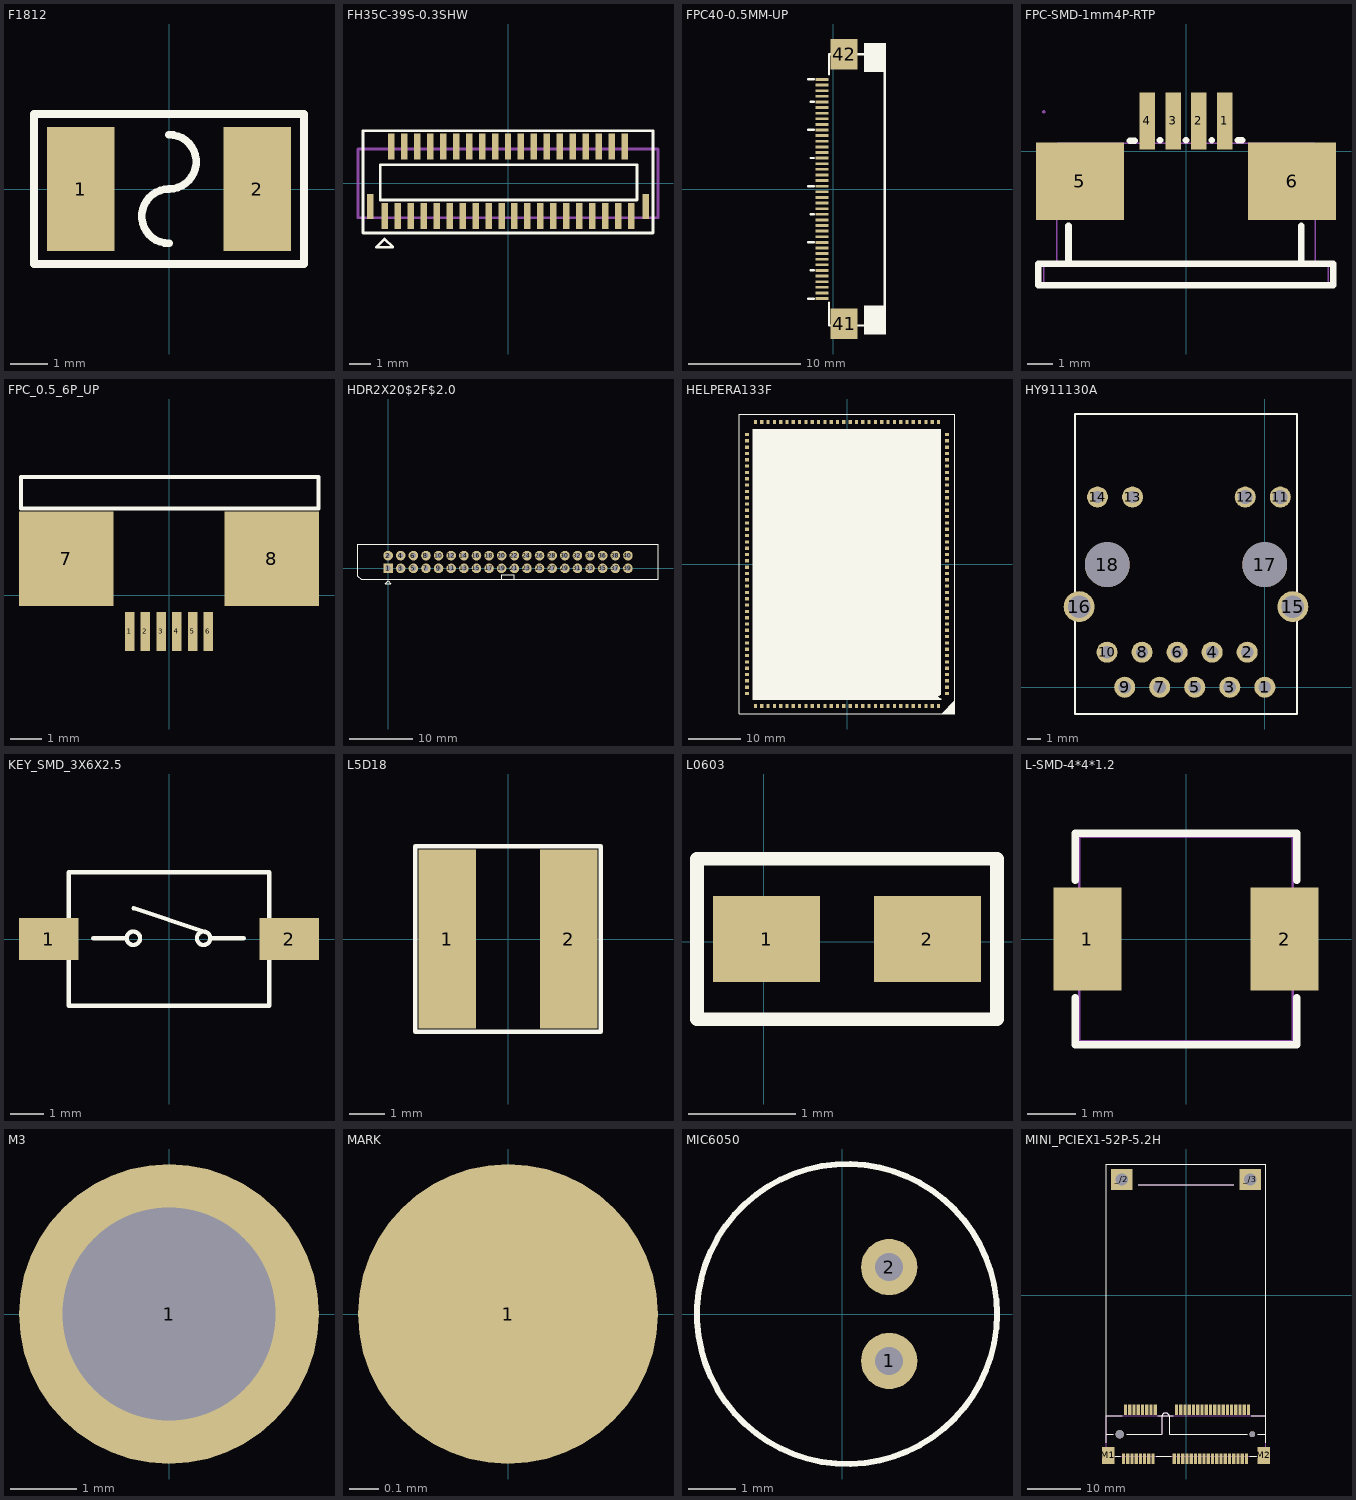
[diagram p0: the footprints below, top view; thin cyan lines are the x and y axes]
# Altium footprint library MISC82162-2.PcbLib: 66 footprints (part 2 of 5)
Each footprint in its own frame and in the unit in brackets; x right, y up, seen from the top. Pads: shape width x height; smd on the part's side, far side on the other; paste and mask are expansions set on the pad; w line width, h text height; cw(c..) or ccw(c..) is an arc to the next point about the centre after c.

## F1812 [mm]
pads (2):
  rect 1.8x3.3 smd: 1(-2.349,0) 2(2.349,0)
Top Overlay:
  lines w0.203: 0,-1.45 cw(c0,-0.725) 0,0 ccw(c0,0.725) 0,1.45 ; -3.6,-2 -3.6,2 3.6,2 3.6,-2 -3.6,-2

## FH35C-39S-0.3SHW [mm]
pads (41):
  rect 0.3x1.2 smd: 1(-5.7,-1.5) 2(-5.4,1.7) 3(-5.1,-1.5) 4(-4.8,1.7) 5(-4.5,-1.5) 6(-4.2,1.7) 7(-3.9,-1.5) 8(-3.6,1.7) 9(-3.3,-1.5) 10(-3,1.7) 11(-2.7,-1.5) 12(-2.4,1.7) 13(-2.1,-1.5) 14(-1.8,1.7) 15(-1.5,-1.5) 16(-1.2,1.7) 17(-0.9,-1.5) 18(-0.6,1.7) 19(-0.3,-1.5) 20(0,1.7) 21(0.3,-1.5) 22(0.6,1.7) 23(0.9,-1.5) 24(1.2,1.7) 25(1.5,-1.5) 26(1.8,1.7) 27(2.1,-1.5) 28(2.4,1.7) 29(2.7,-1.5) 30(3,1.7) 31(3.3,-1.5) 32(3.6,1.7) 33(3.9,-1.5) 34(4.2,1.7) 35(4.5,-1.5) 36(4.8,1.7) 37(5.1,-1.5) 38(5.4,1.7) 39(5.7,-1.5)
  rect 0.3x1.15 smd: 40(6.35,-1.062) 41(-6.35,-1.062)
Top Overlay:
  lines w0.127: -6.7,-2.29 -6.7,2.427 6.7,2.427 6.7,-2.29 -6.7,-2.29 ; -6.08,-2.942 -5.699,-2.561 -5.318,-2.943 -6.068,-2.943 -6.08,-2.942 ; -5.9,-0.768 5.96,-0.768 5.96,0.863 -5.9,0.863 -5.9,-0.768
Mechanical 18:
  lines w0.127: -6.925,-1.587 6.925,-1.587 6.925,1.587 -6.925,1.587 -6.925,-1.587

## FPC40-0.5MM-UP [mm]
pads (42):
  rect 1.15x0.25 smd: 1(-0.984,9.75) 2(-0.984,9.25) 3(-0.984,8.75) 4(-0.984,8.25) 5(-0.984,7.75) 6(-0.984,7.25) 7(-0.984,6.75) 8(-0.984,6.25) 9(-0.984,5.75) 10(-0.984,5.25) 11(-0.984,4.75) 12(-0.984,4.25) 13(-0.984,3.75) 14(-0.984,3.25) 15(-0.984,2.75) 16(-0.984,2.25) 17(-0.984,1.75) 18(-0.984,1.25) 19(-0.984,0.75) 20(-0.984,0.25) 21(-0.984,-0.25) 22(-0.984,-0.75) 23(-0.984,-1.25) 24(-0.984,-1.75) 25(-0.984,-2.25) 26(-0.984,-2.75) 27(-0.984,-3.25) 28(-0.984,-3.75) 29(-0.984,-4.25) 30(-0.984,-4.75) 31(-0.984,-5.25) 32(-0.984,-5.75) 33(-0.984,-6.25) 34(-0.984,-6.75) 35(-0.984,-7.25) 36(-0.984,-7.75) 37(-0.984,-8.25) 38(-0.984,-8.75) 39(-0.984,-9.25) 40(-0.984,-9.75)
  rect 2.4x2.7 smd: 41(0.984,-12) 42(0.984,12)
Top Overlay:
  region: 2.801,-12.924 4.706,-12.924 4.706,-10.384 2.801,-10.384
  region: 2.801,10.444 4.706,10.444 4.706,12.984 2.801,12.984
  lines w0.203: -2.218,-9.761 -1.713,-9.761 ; -2.218,-4.746 -1.713,-4.746 ; -2.218,0.253 -1.713,0.253 ; -2.218,5.262 -1.713,5.262 ; -2.218,9.756 -1.713,9.756 ; -2,-7.241 -1.713,-7.241 ; -2,-2.242 -1.713,-2.242 ; -2,2.767 -1.713,2.767 ; -2,7.769 -1.713,7.769 ; -0.367,-10.106 -0.367,-12.153 4.604,-12.153 4.604,11.992 -0.367,11.992 -0.367,10.189
Top Paste:
  lines w0.152: -0.349,-10.65 -0.349,-12.153 1.316,-12.153

## FPC-SMD-1mm4P-RTP [mm]
pads (6):
  rect 0.6x2.2 smd: 1(1.499,1.163) 2(0.499,1.163) 3(-0.5,1.163) 4(-1.5,1.163)
  rect 3.4x3 smd: 5(-4.1,-1.162) 6(4.1,-1.163)
Top Overlay:
  lines w0.254: -5.718,-5.192 4.48,-5.192 ; -5.718,-5.19 -5.718,-4.36 ; -5.718,-4.352 5.69,-4.352 ; -4.543,-4.352 -4.543,-2.893 ; -2.175,0.4 -1.988,0.4 ; -1.004,0.415 -0.995,0.415 ; -0.004,0.415 0.004,0.415 ; 0.995,0.415 1.004,0.415 ; 1.995,0.415 2.182,0.415 ; 4.456,-4.352 4.456,-2.894 ; 4.49,-5.192 5.69,-5.192 5.69,-4.362
Mechanical 6:
  circle w0.2: c1.525,1.975 r0.1
Mechanical 15:
  region: 5,-2.413 3.2,-2.413 3.2,0.087 5,0.087
  region: -3.2,-2.412 -5,-2.412 -5,0.088 -3.2,0.088
  region: -1.625,1.512 -1.375,1.512 -1.375,0.112 -1.625,0.112
  region: -0.625,1.512 -0.375,1.512 -0.375,0.112 -0.625,0.112
  region: 1.374,1.512 1.624,1.512 1.624,0.112 1.374,0.112
  region: 0.374,1.512 0.625,1.512 0.625,0.112 0.374,0.112
  region: -5.44,1.512 -5.44,1.537 -5.475,1.572 -5.525,1.572 -5.56,1.537 -5.56,1.512 -5.56,1.488 -5.525,1.452 -5.475,1.452 -5.44,1.488
  lines w0.051: -5.5,-5.2 5.5,-5.2 5.5,-4.35 5,-4.35 5,0.3 -5,0.3 -5,-4.325 -5.5,-4.325 -5.5,-5.2

## FPC_0.5_6P_UP [mm]
pads (8):
  rect 0.3x1.25 smd: 1(-1.25,-1.15) 2(-0.75,-1.15) 3(-0.25,-1.15) 4(0.25,-1.15) 5(0.75,-1.15) 6(1.25,-1.15)
  rrect0% 3x3 smd: 7(-3.25,1.15) 8(3.25,1.15)
Top Overlay:
  lines w0.127: -4.691,2.75 4.737,2.75 4.737,3.75 -4.691,3.75 -4.691,2.75

## HDR2X20$2F$2.0 [mil]
pads (40):
  rect 60x60 hole 32: 1(0,0)
  round 60 hole 32: 2(0,78.74) 3(78.74,0) 4(78.74,78.74) 5(157.48,0) 6(157.48,78.74) 7(236.22,0) 8(236.22,78.74) 9(314.96,0) 10(314.96,78.74) 11(393.7,0) 12(393.7,78.74) 13(472.44,0) 14(472.44,78.74) 15(551.18,0) 16(551.18,78.74) 17(629.92,0) 18(629.92,78.74) 19(708.66,0) 20(708.66,78.74) 21(787.4,0) 22(787.4,78.74) 23(866.14,0) 24(866.14,78.74) 25(944.88,0) 26(944.88,78.74) 27(1023.62,0) 28(1023.62,78.74) 29(1102.36,0) 30(1102.36,78.74) 31(1181.1,0) 32(1181.1,78.74) 33(1259.84,0) 34(1259.84,78.74) 35(1338.58,0) 36(1338.58,78.74) 37(1417.32,0) 38(1417.32,78.74) 39(1496.06,0) 40(1496.06,78.74)
Top Overlay:
  lines w5: -0.5,-76.38 18.03,-94.91 -19.02,-94.91 -0.45,-76.34 ; 709.84,-69.69 709.84,-40.16 787.8,-40.16 787.8,-69.69 ; -187.8,-49.69 -167.8,-69.69 1683.86,-69.69 1683.86,148.43 -187.8,148.43 -187.8,-49.69

## HELPERA133F [mm]
pads (144):
  rect 0.8x0.61 smd paste+0.12: 1(19,-24.6) 2(19,-23.4) 3(19,-22.2) 4(19,-21) 5(19,-19.8) 6(19,-18.6) 7(19,-17.4) 8(19,-16.2) 9(19,-15) 10(19,-13.8) 11(19,-12.6) 12(19,-11.4) 13(19,-10.2) 14(19,-9) 15(19,-7.8) 16(19,-6.6) 17(19,-5.4) 18(19,-4.2) 19(19,-3) 20(19,-1.8) 21(19,-0.6) 22(19,0.6) 23(19,1.8) 24(19,3) 25(19,4.2) 26(19,5.4) 27(19,6.6) 28(19,7.8) 29(19,9) 30(19,10.2) 31(19,11.4) 32(19,12.6) 33(19,13.8) 34(19,15) 35(19,16.2) 36(19,17.4) 37(19,18.6) 38(19,19.8) 39(19,21) 40(19,22.2) 41(19,23.4) 42(19,24.6) 73(-19,24.6) 74(-19,23.4) 75(-19,22.2) 76(-19,21) 77(-19,19.8) 78(-19,18.6) 79(-19,17.4) 80(-19,16.2) 81(-19,15) 82(-19,13.8) 83(-19,12.6) 84(-19,11.4) 85(-19,10.2) 86(-19,9) 87(-19,7.8) 88(-19,6.6) 89(-19,5.4) 90(-19,4.2) 91(-19,3) 92(-19,1.8) 93(-19,0.6) 94(-19,-0.6) 95(-19,-1.8) 96(-19,-3) 97(-19,-4.2) 98(-19,-5.4) 99(-19,-6.6) 100(-19,-7.8) 101(-19,-9) 102(-19,-10.2) 103(-19,-11.4) 104(-19,-12.6) 105(-19,-13.8) 106(-19,-15) 107(-19,-16.2) 108(-19,-17.4) 109(-19,-18.6) 110(-19,-19.8) 111(-19,-21) 112(-19,-22.2) 113(-19,-23.4) 114(-19,-24.6)
  rect 0.61x0.8 smd paste+0.12: 43(17.4,27) 44(16.2,27) 45(15,27) 46(13.8,27) 47(12.6,27) 48(11.4,27) 49(10.2,27) 50(9,27) 51(7.8,27) 52(6.6,27) 53(5.4,27) 54(4.2,27) 55(3,27) 56(1.8,27) 57(0.6,27) 58(-0.6,27) 59(-1.8,27) 60(-3,27) 61(-4.2,27) 62(-5.4,27) 63(-6.6,27) 64(-7.8,27) 65(-9,27) 66(-10.2,27) 67(-11.4,27) 68(-12.6,27) 69(-13.8,27) 70(-15,27) 71(-16.2,27) 72(-17.4,27) 115(-17.4,-27) 116(-16.2,-27) 117(-15,-27) 118(-13.8,-27) 119(-12.6,-27) 120(-11.4,-27) 121(-10.2,-27) 122(-9,-27) 123(-7.8,-27) 124(-6.6,-27) 125(-5.4,-27) 126(-4.2,-27) 127(-3,-27) 128(-1.8,-27) 129(-0.6,-27) 130(0.6,-27) 131(1.8,-27) 132(3,-27) 133(4.2,-27) 134(5.4,-27) 135(6.6,-27) 136(7.8,-27) 137(9,-27) 138(10.2,-27) 139(11.4,-27) 140(12.6,-27) 141(13.8,-27) 142(15,-27) 143(16.2,-27) 144(17.4,-27)
Top Overlay:
  region: 17.85,25.6 -17.9,25.6 -17.9,-25.8 17.95,-25.8 17.878,-25.577 17.269,-25.207 17.85,-24.834
  lines w0.127: 18.05,-28.45 20.5,-26 ; 18.3,-28.4 20.5,-26.2 ; 18.4,-28.5 20.45,-26.45 ; 18.6,-28.5 20.4,-26.7 ; 18.9,-28.4 20.4,-26.9 ; 19,-28.5 20.4,-27.1 ; 19.2,-28.4 20.4,-27.2 ; 19.3,-28.4 20.4,-27.3 ; 19.4,-28.5 20.4,-27.5 20.4,-27.4 ; 19.6,-28.4 20.4,-27.6 ; 19.7,-28.4 20.35,-27.75 ; 19.8,-28.4 19.85,-28.45 20.5,-27.8 ; 19.9,-28.5 20.45,-27.95 ; 20.1,-28.4 20.45,-28.05 ; 20.2,-28.5 20.45,-28.25 ; -20.5,-28.5 20.5,-28.5 20.5,28.5 -20.5,28.5 -20.5,-28.5

## HY911130A [mil]
pads (18):
  round 60 hole 35: 1(0,0) 2(-50.39,100) 3(-100,0) 4(-150.39,100) 5(-200,0) 6(-250.39,100) 7(-300,0) 8(-350.39,100) 9(-400,0) 10(-450.39,100) 13(-377.56,542.91) 14(-477.56,542.91)
  round 60 hole 40.16: 11(44.09,542.91) 12(-55.91,542.91)
  round 88.58 / inner round 78.74 / far side round 78.74 hole 64.17: 15(79.92,229.92) 16(-529.92,229.92)
  round 127.95 hole 127.95: 17(0,350) 18(-450,350)
Top Overlay:
  lines w5: -541.93,-76.38 91.93,-76.38 91.93,779.92 -541.93,779.92 -541.93,-76.38

## KEY_SMD_3X6X2.5 [mm]
pads (2):
  rect 1.778x1.27 smd: 1(-3.6,0) 2(3.6,0)
Top Overlay:
  circle w0.127: c1.035,0.023 r0.2
  circle w0.127: c-1.065,0.023 r0.2
  lines w0.127: -2.265,0.023 -1.265,0.023 ; -1.065,0.923 1.035,0.223 ; 1.235,0.023 2.235,0.023 ; -3,-2 3,-2 3,2 -3,2 -3,-2

## L5D18 [mm]
pads (2):
  rect 1.6x5 smd: 1(-1.7,0) 2(1.7,0)
Top Overlay:
  lines w0.127: -2.6,-2.6 -2.6,2.6 2.6,2.6 2.6,-2.6 -2.6,-2.6

## L0603 [mm]
pads (2):
  rect 1x0.8 smd: 1(0.025,0.025) 2(1.525,0.025)
Top Overlay:
  lines w0.127: -0.625,-0.725 -0.625,0.775 2.175,0.775 2.175,-0.725 -0.625,-0.725

## L-SMD-4*4*1.2 [mm]
pads (2):
  rect 1.4x2.12 smd: 1(-2.028,0) 2(2.028,0)
Top Overlay:
  lines w0.152: -2.276,-1.212 -2.276,-2.176 2.276,-2.176 2.276,-1.212 ; -2.276,1.212 -2.276,2.176 2.276,2.176 2.276,1.212
Mechanical 15:
  region: 2.2,-1 1.4,-1 1.4,1 2.2,1
  region: -1.4,-1 -2.2,-1 -2.2,1 -1.4,1
  lines w0.051: -2.2,-2.1 -2.2,2.1 2.2,2.1 2.2,-2.1 -2.2,-2.1

## M3 [mm]
pads (1):
  round 4.5 hole 3.2: 1(0,0)

## MARK [mil]
pads (1):
  round 40 all layers, no hole: 1(0,0)

## MIC6050 [mm]
pads (2):
  round 1.2 hole 0.6: 1(1,-1) 2(1,1)
Top Overlay:
  circle w0.127: c0.1,0 r3.2

## MINI_PCIEX1-52P-5.2H [mm]
pads (58):
  rect 0.61x2.007 smd: 1(-11.8,-30.775) 2(-11.4,-21.575) 3(-11,-30.775) 4(-10.6,-21.575) 5(-10.2,-30.775) 6(-9.8,-21.575) 7(-9.4,-30.775) 8(-9,-21.575) 9(-8.6,-30.775) 10(-8.2,-21.575) 11(-7.8,-30.775) 12(-7.4,-21.575) 13(-7,-30.775) 14(-6.6,-21.575) 15(-6.2,-30.775) 16(-5.8,-21.575) 17(-2.2,-30.775) 18(-1.8,-21.575) 19(-1.4,-30.775) 20(-1,-21.575) 21(-0.6,-30.775) 22(-0.2,-21.575) 23(0.2,-30.775) 24(0.6,-21.575) 25(1,-30.775) 26(1.4,-21.575) 27(1.8,-30.775) 28(2.2,-21.575) 29(2.6,-30.775) 30(3,-21.575) 31(3.4,-30.775) 32(3.8,-21.575) 33(4.2,-30.775) 34(4.6,-21.575) 35(5,-30.775) 36(5.4,-21.575) 37(5.8,-30.775) 38(6.2,-21.575) 39(6.6,-30.775) 40(7,-21.575) 41(7.4,-30.775) 42(7.8,-21.575) 43(8.2,-30.775) 44(8.6,-21.575) 45(9,-30.775) 46(9.4,-21.575) 47(9.8,-30.775) 48(10.2,-21.575) 49(10.6,-30.775) 50(11,-21.575) 51(11.4,-30.775) 52(11.8,-21.575)
  rect 4x4 / inner round 4 / far side rect 4x4 hole 2.3: _/2(-12.1,21.875) _/3(12.1,21.875)
  round 1.6 hole 1.6: G1(-12.5,-26.175)
  round 1.092 hole 1.092: G2(12.5,-26.175)
  rect 2.311x3.2 smd: M1(-14.65,-30.175) M2(14.65,-30.175)
Top Overlay:
  lines w0.152: -15,-27.775 -15,24.775 15,24.775 15,-27.775 ; -15,-26.175 -13.7,-26.175 ; -15,-22.675 -12,-22.675 ; -13.3,-30.275 -12.4,-30.275 ; -11.2,-26.175 -4.6,-26.175 -4.6,-22.925 cw(c-3.85,-22.925) -3.1,-22.925 -3.1,-26.175 11.5,-26.175 ; -9,20.825 9,20.825 ; -5.6,-30.275 -2.8,-30.275 ; -5.3,-22.675 -2.4,-22.675 ; 12,-30.275 13.3,-30.275 ; 12.3,-22.675 15,-22.675 ; 13.5,-26.175 15,-26.175
Top Paste:
  region: 10,19.775 14.2,19.775 14.2,23.975 10,23.975
  region: -14.2,19.775 -10,19.775 -10,23.975 -14.2,23.975
  region: -14.15,19.825 -10.05,19.825 -10.05,23.925 -14.15,23.925
Mechanical 12:
  lines w0.152: -15,-26.175 -13.7,-26.175 ; -15,-22.675 -12,-22.675 ; -13.3,-30.275 -12.4,-30.275 ; -11.2,-26.175 -4.6,-26.175 -4.6,-22.925 cw(c-3.85,-22.925) -3.1,-22.925 -3.1,-26.175 11.5,-26.175 ; -9,20.825 9,20.825 ; -5.6,-30.275 -2.8,-30.275 ; -5.3,-22.675 -2.4,-22.675 ; 12,-30.275 13.3,-30.275 ; 12.3,-22.675 15,-22.675 ; 13.5,-26.175 15,-26.175 ; 15,-27.775 15,-5.147
Mechanical 13:
  lines w0.025: -15,-30.275 15,-30.275 15,-22.675 -15,-22.675 -15,-30.275